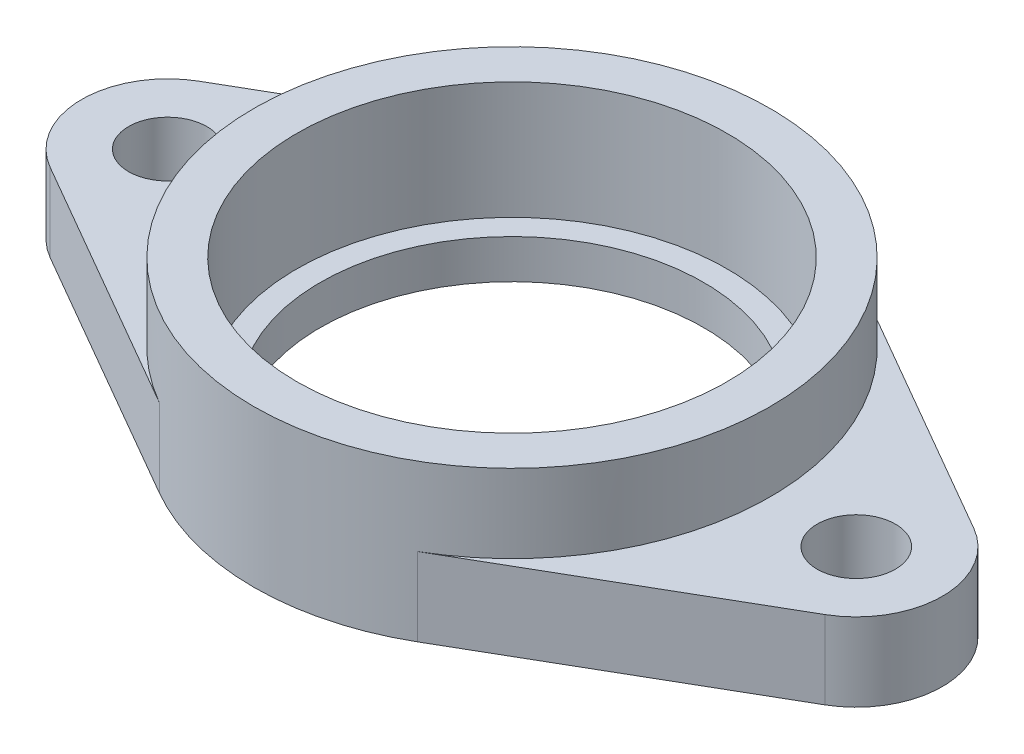
SolidWorks part; units mm, degrees
ref_plane "前视基准面" through (0, 0, 0) normal (0, 0, 1) x (1, 0, 0)
ref_plane "上视基准面" through (0, 0, 0) normal (0, 1, 0) x (1, 0, 0)
ref_plane "右视基准面" through (0, 0, 0) normal (1, 0, 0) x (0, 0, -1)
sketch "草图1" plane through (0, 0, 0) normal (0, 1, 0) x (1, 0, 0)
  line L0 (-49.5, 9.5263) -> (-16.5, 28.5788)
  line L1 (16.5, 28.5788) -> (49.5, 9.5263)
  line L2 (49.5, -9.5263) -> (16.5, -28.5788)
  line L3 (-16.5, -28.5788) -> (-49.5, -9.5263)
  arc A0 (-16.5, -28.5788) -> (16.5, -28.5788) centre (0, 0) ccw
  arc A1 (49.5, -9.5263) -> (49.5, 9.5263) centre (44, 0) ccw
  arc A2 (-49.5, 9.5263) -> (-49.5, -9.5263) centre (-44, 0) ccw
  arc A3 (16.5, 28.5788) -> (-16.5, 28.5788) centre (0, 0) ccw
  circle A4 centre (-44, 0) radius 5
  circle A5 centre (44, 0) radius 5
  dimension "D1" = 44
  dimension "D2" = 44
extrude "凸台-拉伸1" add sketch "草图1" along normal blind 10
sketch "草图2" plane through (0, 10, 0) normal (0, 1, 0) x (1, 0, 0)
  circle A0 centre (0, 0) radius 33
extrude "凸台-拉伸2" add sketch "草图2" along normal blind 10
sketch "草图3" plane through (0, 20, 0) normal (0, 1, 0) x (1, 0, 0)
  circle A0 centre (0, 0) radius 27.5
extrude "切除-拉伸1" cut sketch "草图3" against normal blind 15
sketch "草图4" plane through (0, 5, 0) normal (0, 1, 0) x (1, 0, 0)
  circle A0 centre (0, 0) radius 24.5
extrude "切除-拉伸2" cut sketch "草图4" against normal blind 15
